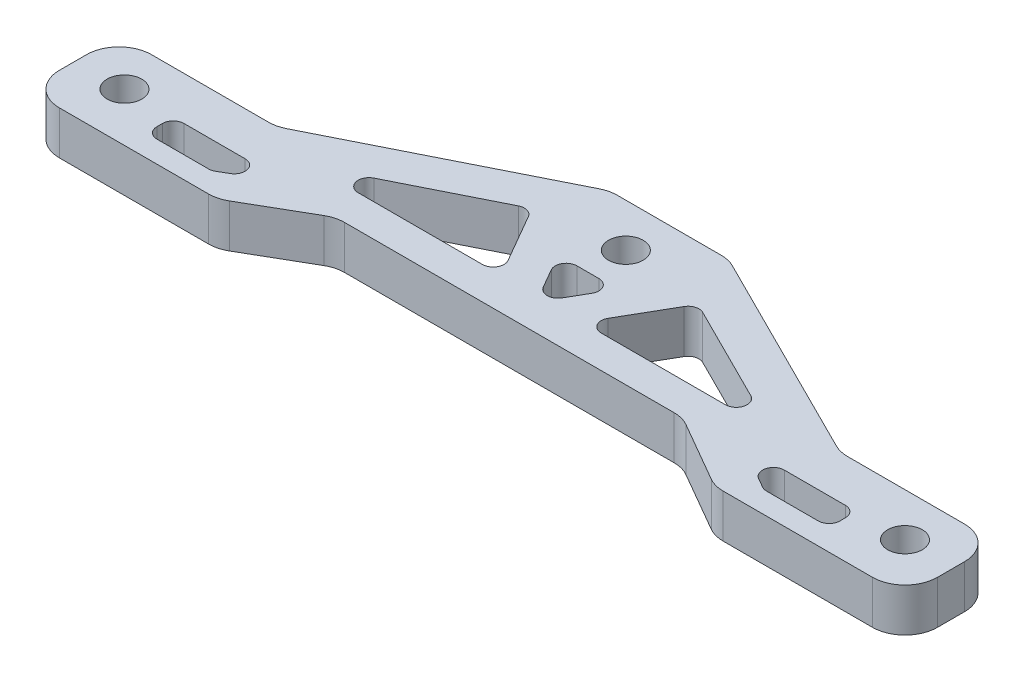
from build123d import *

# Parameters (mm, degrees)
SKETCH1_R              = 1.6
BOSS_EXTRUDE1_DEPTH    = 4
CUT_EXTRUDE1_DEPTH     = 44.119746057
R1_CUTOUT_FILLET_R     = 1
R3_OUTER_EDGE_FILLET_R = 3


with BuildPart() as part:
    # Sketch1 → Boss-Extrude1 (new body)
    with BuildSketch(Plane(origin=(0, 0, 0), x_dir=(1, 0, 0), z_dir=(0, 1, 0))):
        Polygon((-40.5, -4.5), (-22.92820323, -4.5), (-16, -0.5), (16, -0.5), (22.92820323, -4.5), (40.5, -4.5), (40.5, 4), (26, 4), (5.5, 14.25), (-5.5, 14.25), (-26, 4), (-40.5, 4), align=None)
        with Locations(Location((-36, 0, 0), (0, 0, 270))):
            Circle(SKETCH1_R, mode=Mode.SUBTRACT)
        with Locations(Location((36, 0, 0), (0, 0, 270))):
            Circle(SKETCH1_R, mode=Mode.SUBTRACT)
        with Locations(Location((0, 10.25, 0), (0, 0, 270))):
            Circle(SKETCH1_R, mode=Mode.SUBTRACT)
    extrude(amount=BOSS_EXTRUDE1_DEPTH)

    # Sketch2 → Cut-Extrude1 (cut, through all)
    with BuildSketch(Plane(origin=(0, 4, 0), x_dir=(1, 0, 0), z_dir=(0, 1, 0))):
        Polygon((-7.655238394, 9.259261842), (-21.173762079, 2.5), (-3.75277675, 2.5), align=None)
        Polygon((-2.742413779, 6.75), (0, 2), (2.742413779, 6.75), align=None)
        Polygon((21.173762079, 2.5), (3.75277675, 2.5), (7.655238394, 9.259261842), align=None)
        Polygon((-31.5, 0), (-21.133974596, 0), (-25.464101615, -2.5), (-31.5, -2.5), align=None)
        Polygon((25.464101615, -2.5), (31.5, -2.5), (31.5, 0), (21.133974596, 0), align=None)
    extrude(amount=-CUT_EXTRUDE1_DEPTH, mode=Mode.SUBTRACT)

    # R1 cutout fillet
    r1_cutout_fillet_edges = [part.edges().sort_by_distance(p)[0] for p in [
        (-25.464101615, 2, 2.5),
        (-31.5, 2, 2.5),
        (-31.5, 2, 0),
        (-21.133974596, 2, 0),
        (25.464101615, 2, 2.5),
        (21.133974596, 2, 0),
        (31.5, 2, 0),
        (31.5, 2, 2.5),
        (7.655238394, 2, -9.259261842),
        (21.173762079, 2, -2.5),
        (3.75277675, 2, -2.5),
        (-2.742413779, 2, -6.75),
        (2.742413779, 2, -6.75),
        (0, 2, -2),
        (-7.655238394, 2, -9.259261842),
        (-3.75277675, 2, -2.5),
        (-21.173762079, 2, -2.5),
    ]]
    fillet(r1_cutout_fillet_edges, radius=R1_CUTOUT_FILLET_R)

    # R3 outer edge fillet
    r3_outer_edge_fillet_edges = [part.edges().sort_by_distance(p)[0] for p in [
        (40.5, 2, -4),
        (40.5, 2, 4.5),
        (22.92820323, 2, 4.5),
        (16, 2, 0.5),
        (-16, 2, 0.5),
        (-22.92820323, 2, 4.5),
        (-40.5, 2, 4.5),
        (-40.5, 2, -4),
        (-26, 2, -4),
        (-5.5, 2, -14.25),
        (5.5, 2, -14.25),
        (26, 2, -4),
    ]]
    fillet(r3_outer_edge_fillet_edges, radius=R3_OUTER_EDGE_FILLET_R)


solid = part.part
